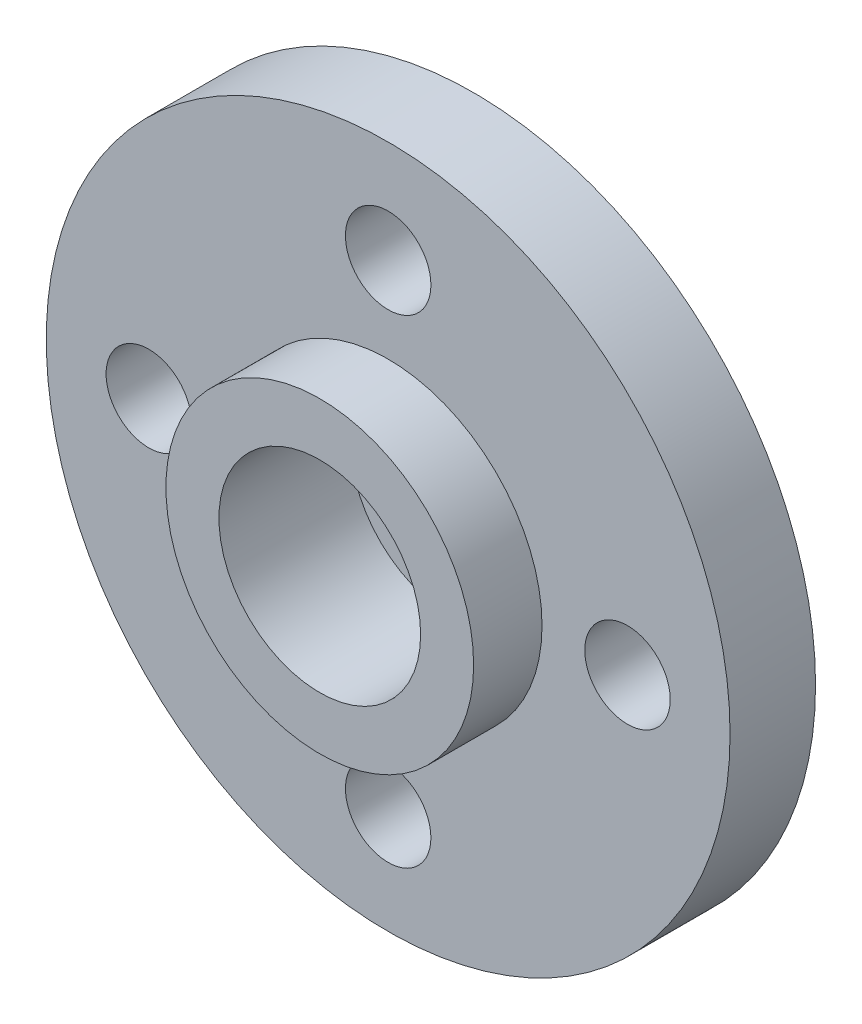
from build123d import *

# Parameters (mm, degrees)
SKETCH1_R           = 10
BOSS_EXTRUDE1_DEPTH = 4.5
CUT_EXTRUDE1_START  = -2
SKETCH2_R           = 10
SKETCH2_R_2         = 4.5
CUT_EXTRUDE1_DEPTH  = 2
SKETCH3_R           = 0.75
CUT_EXTRUDE2_DEPTH  = 15.361406616
SKETCH4_R           = 2.95
CUT_EXTRUDE3_DEPTH  = 3.85
SKETCH5_R           = 1.5
CUT_EXTRUDE4_DEPTH  = 15.656824349
M3_TAPPED_HOLE2_D   = 2.5


with BuildPart() as part:
    # Sketch1 → Boss-Extrude1 (new body)
    with BuildSketch(Plane.XY):
        Circle(SKETCH1_R)
    extrude(amount=BOSS_EXTRUDE1_DEPTH)

    # Sketch2 → Cut-Extrude1 (cut)
    with BuildSketch(Plane.XY.offset(4.5).offset(CUT_EXTRUDE1_START)):
        Circle(SKETCH2_R)
        Circle(SKETCH2_R_2, mode=Mode.SUBTRACT)
    extrude(amount=CUT_EXTRUDE1_DEPTH, mode=Mode.SUBTRACT)

    # Sketch3 → Cut-Extrude2 (cut, through all)
    with BuildSketch(Plane.XY.offset(2.5)):
        with Locations((0, 7)):
            Circle(SKETCH3_R)
        with Locations((7, 0)):
            Circle(SKETCH3_R)
        with Locations((0, -7)):
            Circle(SKETCH3_R)
        with Locations((-7, 0)):
            Circle(SKETCH3_R)
    extrude(amount=-CUT_EXTRUDE2_DEPTH, mode=Mode.SUBTRACT)

    # Sketch4 → Cut-Extrude3 (cut)
    with BuildSketch(Plane.XY.offset(4.5)):
        Circle(SKETCH4_R)
    extrude(amount=-CUT_EXTRUDE3_DEPTH, mode=Mode.SUBTRACT)

    # Sketch5 → Cut-Extrude4 (cut, through all)
    with BuildSketch(Plane.XY.offset(0.65)):
        Circle(SKETCH5_R)
    extrude(amount=-CUT_EXTRUDE4_DEPTH, mode=Mode.SUBTRACT)

    # M3 Tapped Hole2 (through all)
    with Locations(Plane.XY.offset(2.5)):
        with Locations((-7, 0), (0, 7), (7, 0), (0, -7)):
            Hole(M3_TAPPED_HOLE2_D / 2)


solid = part.part
